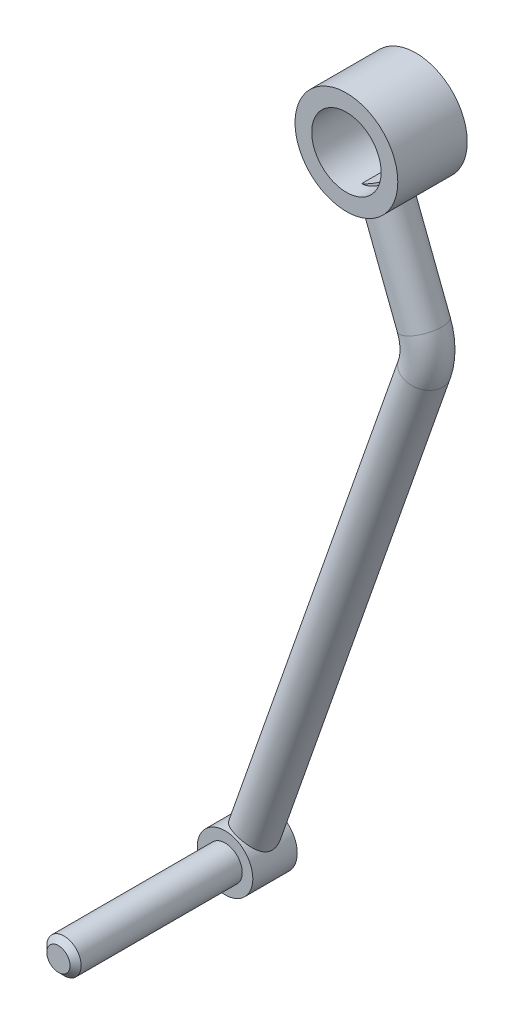
from build123d import *

# Parameters (mm, degrees)
SKETCH1_R           = 9.25
SKETCH1_R_2         = 6.25
BOSS_EXTRUDE1_DEPTH = 12.5
SWEEP1_PROFILE_R    = 3.5
SKETCH16_R          = 5
BOSS_EXTRUDE2_DEPTH = 4
SKETCH17_R          = 3.096104317
BOSS_EXTRUDE3_DEPTH = 30
CHAMFER1_SIZE       = 1


with BuildPart() as part:
    # Sketch1 → Boss-Extrude1 (new body)
    with BuildSketch(Plane.XY):
        Circle(SKETCH1_R)
        Circle(SKETCH1_R_2, mode=Mode.SUBTRACT)
    extrude(amount=BOSS_EXTRUDE1_DEPTH)

    # Sweep1: sweep along a curve in space
    with BuildLine() as sweep1_path:
        Line((0, -6.25, 6.25), (7.675401854, -26.137831295, 6.25))
        ThreePointArc((7.782428128, -33.048212427, 6.25), (8.344876366, -29.583482004, 6.25), (7.675401854, -26.137831295, 6.25))
        Line((7.782428128, -33.048212427, 6.25), (-24.097440523, -123.936842128, 6.25))
    # Sweep1 profile (on start of the path) → Sweep1 (sweep)
    with BuildSketch(Plane(origin=(0, -6.25, 6.25), x_dir=(-0.9329326350915154, -0.36005096636615397, 0), z_dir=(0.36005096636615397, -0.9329326350915154, 0))):
        Circle(SWEEP1_PROFILE_R)
    sweep(path=sweep1_path.line)

    # Sketch16 → Boss-Extrude2 (add, symmetric)
    with BuildSketch(Plane.XY.offset(6.25)):
        with Locations((-24.097440523, -123.936842128)):
            Circle(SKETCH16_R)
    extrude(amount=BOSS_EXTRUDE2_DEPTH, both=True)

    # Sketch17 → Boss-Extrude3 (add)
    with BuildSketch(Plane.XY.offset(10.25)):
        with Locations((-24.097440523, -123.936842128)):
            Circle(SKETCH17_R)
    extrude(amount=BOSS_EXTRUDE3_DEPTH)

    # Chamfer1
    chamfer1_edges = [part.edges().sort_by_distance(p)[0] for p in [
        (-27.19354484, -123.936842128, 40.25),
    ]]
    chamfer(chamfer1_edges, length=CHAMFER1_SIZE)


solid = part.part
